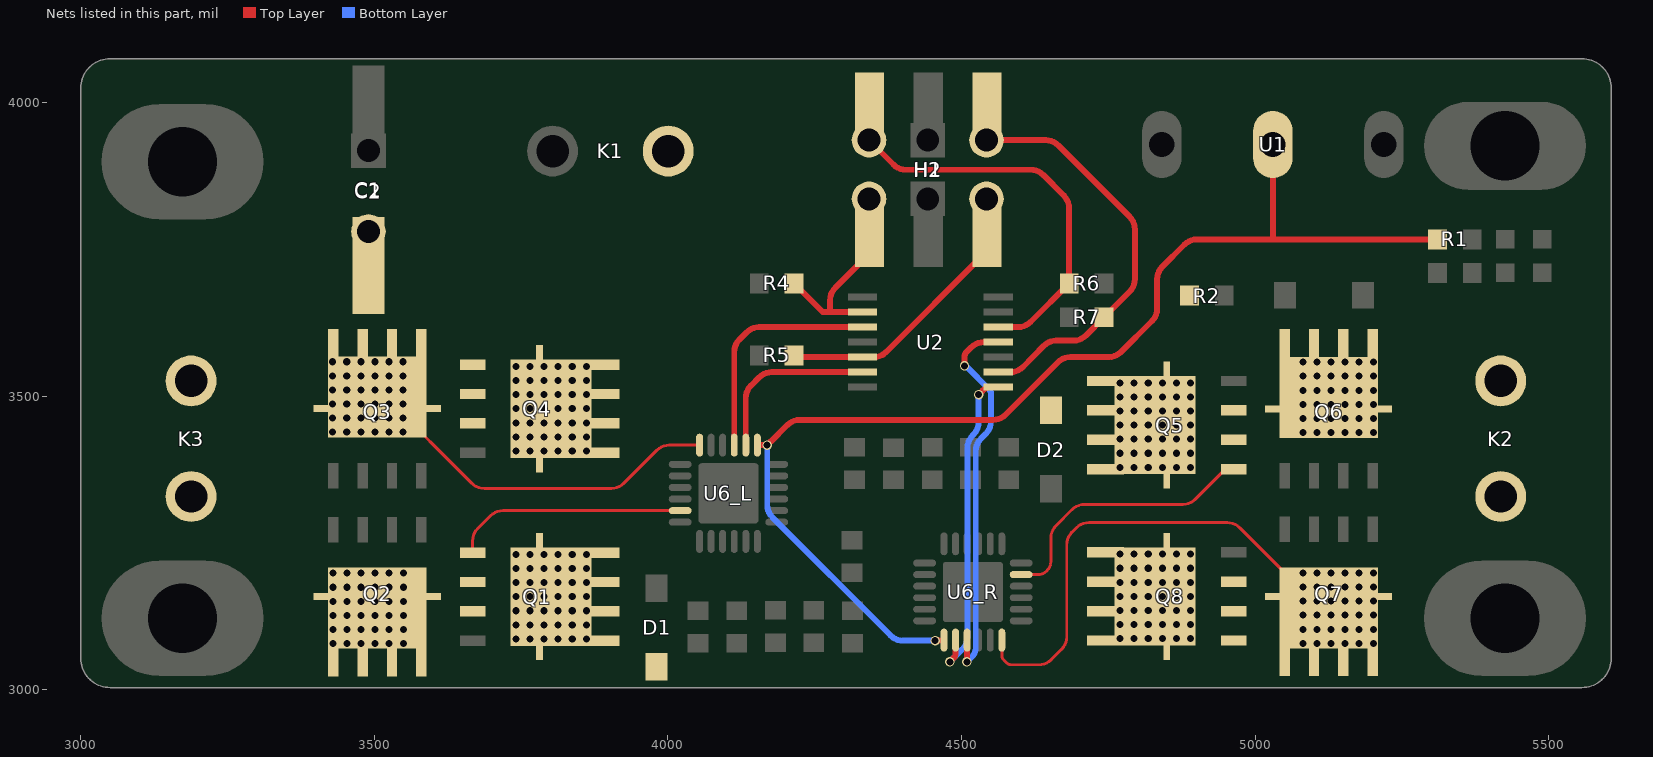
[diagram p0: the nets of this part, all layers, seen from the top]
# Altium PCB MISC62357.pcbdoc (part 2 of 2)
Units mil, origin at the board's own origin, x right, y up, seen from the top; angles counter-clockwise.
Board outline 2606.3 x 1070.87 mil, 2 copper layers (Top Layer, Bottom Layer), stack 62.206 mil thick; 46 components, 37 nets, 219 pads, 514 vias.

## Via types
v1: diameter 16, hole 12, Top Layer to Bottom Layer, 514 vias

## Nets (pads, with @x,y where several pads share a name; then routed paths per layer and width w, separated by ;. In a path a pad name is that pad's centre, name@x,y a point inside that pad or via, vN(x,y) a via of type N, cw(c..) or ccw(c..) an arc to the next point about the centre after c; other vN are vias at no path point) (continued)
L_A: K3.2 Q1.3 Q2.1 U6_L.23 | length 399.4
  Top Layer w5: Q1.3@3667.31,3233.6 3667.31,3253.49 cw(c3697.31,3253.49) 3676.1,3274.7 3697.69,3296.29 cw(c3718.9,3275.08) 3718.9,3305.08 U6_L.23@4020.8,3305.08
  other v1: 3429.35,3078.6 3453.35,3078.6 3477.35,3078.6 3501.35,3078.6 3525.35,3078.6 3549.35,3078.6 3429.35,3102.6 3453.35,3102.6 3477.35,3102.6 3501.35,3102.6 3525.35,3102.6 3549.35,3102.6 3429.35,3126.6 3453.35,3126.6 3477.35,3126.6 3501.35,3126.6 3525.35,3126.6 3549.35,3126.6 3429.35,3150.6 3453.35,3150.6 3477.35,3150.6 3501.35,3150.6 3525.35,3150.6 3549.35,3150.6 3429.35,3174.6 3453.35,3174.6 3477.35,3174.6 3501.35,3174.6 3525.35,3174.6 3549.35,3174.6 3429.35,3198.6 3453.35,3198.6 3477.35,3198.6 3501.35,3198.6 3525.35,3198.6 3549.35,3198.6
L_B: K3.1 Q3.1 Q4.3 U6_L.18 | length 639.5
  Top Layer w5: Q3.1@3505,3498.29 3515.17,3498.29 cw(c3515.17,3488.29) 3522.24,3495.36 3666.03,3351.57 ccw(c3687.24,3372.79) 3687.24,3342.79 3903.51,3342.79 ccw(c3903.51,3372.79) 3924.72,3351.57 3980.92,3407.77 cw(c4002.13,3386.56) 4002.13,3416.56 U6_L.18@4053.79,3416.56
  other v1: 3429,3438.6 3453,3438.6 3477,3438.6 3501,3438.6 3525,3438.6 3549,3438.6 3429,3462.6 3453,3462.6 3477,3462.6 3501,3462.6 3525,3462.6 3549,3462.6 3429,3486.6 3453,3486.6 3477,3486.6 3501,3486.6 3525,3486.6 3549,3486.6 3429,3510.6 3453,3510.6 3477,3510.6 3501,3510.6 3525,3510.6 3549,3510.6 3429,3534.6 3453,3534.6 3477,3534.6 3501,3534.6 3525,3534.6 3549,3534.6 3429,3558.6 3453,3558.6 3477,3558.6 3501,3558.6 3525,3558.6 3549,3558.6
L_DIR_IN: H1.1 H2.1 R4.1 U2.2 | length 294.4
  Top Layer w10: R4.1@4214.66,3692.07 4263.53,3643.21 4275.95,3643.21 ; U2.2@4331.32,3643.21 4275.95,3643.21 ; H1.1@4343.16,3775.44 4343.16,3755.18 cw(c4313.16,3755.18) 4334.37,3733.97 4284.74,3684.34 ccw(c4305.95,3663.13) 4275.95,3663.13 4275.95,3643.21
L_DIR_O: U2.3 U6_L.15 | length 399.3
  Top Layer w10: U6_L.15@4112.84,3416.56 4112.84,3575.01 cw(c4142.84,3575.01) 4121.63,3596.23 4134.23,3608.83 cw(c4155.44,3587.62) 4155.44,3617.62 U2.3@4331.32,3617.62
L_PWM_IN: H1.5 H2.5 R5.1 U2.5 | length 429.2
  Top Layer w10: R5.1@4214.73,3566.44 U2.5@4331.32,3566.44 4350.41,3566.44 ccw(c4350.41,3596.44) 4371.62,3575.22 4534.37,3737.97 ccw(c4513.16,3759.18) 4543.16,3759.18 H1.5@4543.16,3775.44
L_PWM_O: U2.6 U6_L.14 | length 301.9
  Top Layer w10: U6_L.14@4132.53,3416.56 4132.53,3496.7 cw(c4162.53,3496.7) 4141.32,3517.92 4155.46,3532.06 cw(c4176.67,3510.85) 4176.67,3540.85 U2.6@4331.32,3540.85
PWR_EN: R1.2 U1.2 U6_L.13 U6_R.13 | length 2002.7
  Top Layer w10: U6_L.13@4152.25,3416.6 4160.72,3416.6 ccw(c4160.72,3436.6) 4168.37,3418.12 ccw(c4160.72,3436.6) 4174.86,3422.46 4203.21,3450.81 cw(c4224.43,3429.6) 4224.43,3459.6 4553.57,3459.6 ccw(c4553.57,3489.6) 4574.79,3468.39 4664.21,3557.81 cw(c4685.43,3536.6) 4685.43,3566.6 4750.57,3566.6 ccw(c4750.57,3596.6) 4771.79,3575.39 4824.21,3627.81 ccw(c4803,3649.03) 4833,3649.03 4833,3699.17 cw(c4863,3699.17) 4841.79,3720.39 4879.5,3758.1 cw(c4900.72,3736.89) 4900.72,3766.89 5029.26,3766.89 ; v1(4455,3083.6) 4468.99,3083.6 U6_R.13@4470.03,3084.64 ; U1.2@5030.01,3928.47 5030.01,3767.63 5029.26,3766.89 ; R1.2@5310.34,3766.89 5029.26,3766.89
  Bottom Layer w10: v1(4169,3416.6) 4169,3315.03 ccw(c4199,3315.03) 4177.79,3293.81 4379.21,3092.39 ccw(c4400.43,3113.6) 4400.43,3083.6 v1(4455,3083.6)
R_A: K2.2 Q5.3 Q6.1 U6_R.23 | length 466.2
  Top Layer w5: U6_R.23@4601.44,3196.12 4630.24,3196.12 ccw(c4630.24,3216.12) 4644.38,3201.98 4646.13,3203.73 ccw(c4631.98,3217.87) 4651.98,3217.87 4651.98,3258.23 cw(c4681.98,3258.23) 4660.77,3279.44 4688.14,3306.81 cw(c4709.35,3285.6) 4709.35,3315.6 4876.57,3315.6 ccw(c4876.57,3345.6) 4897.79,3324.39 4946.23,3372.83 cw(c4953.3,3365.76) 4953.3,3375.76 Q5.3@4963.47,3375.76
  other v1: 5081,3437.97 5105,3437.97 5129,3437.97 5153,3437.97 5177,3437.97 5201,3437.97 5081,3461.97 5105,3461.97 5129,3461.97 5153,3461.97 5177,3461.97 5201,3461.97 5081,3485.97 5105,3485.97 5129,3485.97 5153,3485.97 5177,3485.97 5201,3485.97 5081,3509.97 5105,3509.97 5129,3509.97 5153,3509.97 5177,3509.97 5201,3509.97 5081,3533.97 5105,3533.97 5129,3533.97 5153,3533.97 5177,3533.97 5201,3533.97 5081,3557.97 5105,3557.97 5129,3557.97 5153,3557.97 5177,3557.97 5201,3557.97
R_B: K2.1 Q7.1 Q8.3 U6_R.18 | length 851.2
  Top Layer w5: U6_R.18@4568.45,3084.64 4568.45,3058.29 ccw(c4578.45,3058.29) 4571.38,3051.22 4577.06,3045.55 ccw(c4584.13,3052.62) 4584.13,3042.62 4631.59,3042.62 ccw(c4631.59,3072.62) 4652.8,3051.4 4670.24,3068.84 ccw(c4649.03,3090.06) 4679.03,3090.06 4679.03,3247.03 cw(c4709.03,3247.03) 4687.82,3268.24 4695.52,3275.94 cw(c4716.74,3254.73) 4716.74,3284.73 4952.44,3284.73 cw(c4952.44,3254.73) 4973.66,3275.94 4973.66,3275.75 5107.2,3142.21 5107.39,3142.21 ccw(c5114.47,3149.28) 5114.47,3139.28 Q7.1@5125,3139.28
  other v1: 5081,3078.96 5105,3078.96 5129,3078.96 5153,3078.96 5177,3078.96 5201,3078.96 5081,3102.96 5105,3102.96 5129,3102.96 5153,3102.96 5177,3102.96 5201,3102.96 5081,3126.96 5105,3126.96 5129,3126.96 5153,3126.96 5177,3126.96 5201,3126.96 5081,3150.96 5105,3150.96 5129,3150.96 5153,3150.96 5177,3150.96 5201,3150.96 5081,3174.96 5105,3174.96 5129,3174.96 5153,3174.96 5177,3174.96 5201,3174.96 5081,3198.96 5105,3198.96 5129,3198.96 5153,3198.96 5177,3198.96 5201,3198.96
R_DIR_IN: H1.2 H2.2 R6.2 U2.12 | length 671.2
  Top Layer w10: H2.2@4342.39,3935.88 4383.88,3894.39 ccw(c4405.1,3915.6) 4405.1,3885.6 4617.57,3885.6 cw(c4617.57,3855.6) 4638.79,3876.81 4674.21,3841.39 cw(c4653,3820.17) 4683,3820.17 4683,3692.2 R6.2@4683.13,3692.07 4617.47,3626.4 cw(c4596.26,3647.62) 4596.26,3617.62 U2.12@4561.64,3617.62
R_DIR_O: U2.11 U6_R.15 | length 657.9
  Top Layer w10: v1(4505,3551.6) 4505,3567.46 cw(c4515,3567.46) 4507.93,3574.53 4516.64,3583.24 cw(c4537.85,3562.03) 4537.85,3592.03 U2.11@4561.64,3592.03 ; v1(4509,3047.6) 4509,3084.24 U6_R.15@4509.4,3084.64
  Bottom Layer w10: v1(4505,3551.6) 4506.87,3551.6 4548,3510.47 4548,3508.6 4550,3506.6 4550,3457.03 cw(c4520,3457.03) 4541.21,3435.81 4532.79,3427.39 ccw(c4554,3406.17) 4524,3406.17 4524,3070.88 cw(c4504,3070.88) 4518.14,3056.74 v1(4509,3047.6)
R_PWM_IN: H1.6 H2.6 R7.2 U2.9 | length 709.1
  Top Layer w10: H2.6@4542.39,3935.88 4643.29,3935.88 cw(c4643.29,3905.88) 4664.51,3927.09 4786.21,3805.39 cw(c4765,3784.17) 4795,3784.17 4795,3699.34 cw(c4765,3699.34) 4786.21,3678.13 R7.2@4744.34,3636.26 ; U2.9@4561.64,3540.85 4583.15,3540.85 ccw(c4583.15,3570.85) 4604.51,3549.78 4639.9,3585.67 cw(c4661.26,3564.6) 4661.26,3594.6 4690.71,3594.6 ccw(c4690.71,3624.6) 4712.07,3603.53 R7.2@4742.45,3634.37 ; R7.2@4742.45,3634.37 R7.2@4744.34,3636.26 ; R7.2@4742.45,3634.37 R7.2@4744.34,3636.26
R_PWM_O: U2.8 U6_R.14 | length 549.1
  Top Layer w10: v1(4480,3047.6) 4486.78,3054.38 ccw(c4479.71,3061.45) 4489.71,3061.45 U6_R.14@4489.71,3084.64 ; v1(4529,3502.6) 4535.8,3509.4 cw(c4549.94,3495.26) 4549.94,3515.26 U2.8@4561.64,3515.26
  Bottom Layer w10: v1(4480,3047.6) 4501.2,3068.8 ccw(c4479.98,3090.01) 4509.98,3090.01 4509.98,3411.98 cw(c4539.98,3411.98) 4518.77,3433.19 4520.21,3434.63 ccw(c4499,3455.85) 4529,3455.85 v1(4529,3502.6)
VM: C1.1 C2.1 D1.2 D2.2 K1.1 Q1.1 Q4.1 Q5.1 Q8.1 R2.2
  other v1: 3741,3086.6 3765,3086.6 3789,3086.6 3813,3086.6 3837,3086.6 3861,3086.6 4769.79,3086.96 4793.79,3086.96 4817.79,3086.96 4841.79,3086.96 4865.79,3086.96 4889.79,3086.96 3741,3110.6 3765,3110.6 3789,3110.6 3813,3110.6 3837,3110.6 3861,3110.6 4769.79,3110.96 4793.79,3110.96 4817.79,3110.96 4841.79,3110.96 4865.79,3110.96 4889.79,3110.96 3741,3134.6 3765,3134.6 3789,3134.6 3813,3134.6 3837,3134.6 3861,3134.6 4769.79,3134.96 4793.79,3134.96 4817.79,3134.96 4841.79,3134.96 4865.79,3134.96 4889.79,3134.96 3741,3158.6 3765,3158.6 3789,3158.6 3813,3158.6 3837,3158.6 3861,3158.6 4769.79,3158.96 4793.79,3158.96 4817.79,3158.96 4841.79,3158.96 4865.79,3158.96 4889.79,3158.96 3741,3182.6 3765,3182.6 3789,3182.6 3813,3182.6 3837,3182.6 3861,3182.6 4769.79,3182.96 4793.79,3182.96 4817.79,3182.96 4841.79,3182.96 4865.79,3182.96 4889.79,3182.96 3741,3206.6 3765,3206.6 3789,3206.6 3813,3206.6 3837,3206.6 3861,3206.6 4769.79,3206.96 4793.79,3206.96 4817.79,3206.96 4841.79,3206.96 4865.79,3206.96 4889.79,3206.96 3741,3230.6 3765,3230.6 3789,3230.6 3813,3230.6 3837,3230.6 3861,3230.6 4769.79,3230.96 4793.79,3230.96 4817.79,3230.96 4841.79,3230.96 4865.79,3230.96 4889.79,3230.96 4769.79,3378.76 4793.79,3378.76 4817.79,3378.76 4841.79,3378.76 4865.79,3378.76 4889.79,3378.76 4769.79,3402.76 4793.79,3402.76 4817.79,3402.76 4841.79,3402.76 4865.79,3402.76 4889.79,3402.76 3741,3406.6 3765,3406.6 3789,3406.6 3813,3406.6 3837,3406.6 3861,3406.6 4769.79,3426.76 4793.79,3426.76 4817.79,3426.76 4841.79,3426.76 4865.79,3426.76 4889.79,3426.76 3741,3430.6 3765,3430.6 3789,3430.6 3813,3430.6 3837,3430.6 3861,3430.6 4769.79,3450.76 4793.79,3450.76 4817.79,3450.76 4841.79,3450.76 4865.79,3450.76 4889.79,3450.76 3741,3454.6 3765,3454.6 3789,3454.6 3813,3454.6 3837,3454.6 3861,3454.6 4769.79,3474.76 4793.79,3474.76 4817.79,3474.76 4841.79,3474.76 4865.79,3474.76 4889.79,3474.76 3741,3478.6 3765,3478.6 3789,3478.6 3813,3478.6 3837,3478.6 3861,3478.6 4769.79,3498.76 4793.79,3498.76 4817.79,3498.76 4841.79,3498.76 4865.79,3498.76 4889.79,3498.76 3741,3502.6 3765,3502.6 3789,3502.6 3813,3502.6 3837,3502.6 3861,3502.6 4769.79,3522.76 4793.79,3522.76 4817.79,3522.76 4841.79,3522.76 4865.79,3522.76 4889.79,3522.76 3741,3526.6 3765,3526.6 3789,3526.6 3813,3526.6 3837,3526.6 3861,3526.6 3741,3550.6 3765,3550.6 3789,3550.6 3813,3550.6 3837,3550.6 3861,3550.6
pads on no net: U6_L.9 U6_L.10 U6_L.11 U6_R.9 U6_R.10 U6_R.11

## Polygon pours and split planes (outlines as drawn)
VM on Top Layer (solid, remove dead copper, pour order 16): 3888.79,3989.85 3888.79,3714.75 4098.85,3714.75 4098.85,3989.85
VM on Bottom Layer (solid, remove dead copper, pour order 32): 3433,3830.6 3433,3739.6 3809,3739.6 3809,3830.6
VM on Bottom Layer (solid, remove dead copper, pour order 34): 3888.79,3989.85 3888.79,3730.75 4098.85,3730.75 4098.85,3989.85
VM on Top Layer (solid, remove dead copper, pour order 0): 3368.4,3830.59 3368.4,3644.33 3705.15,3644.33 3705.15,3393.67 3925.27,3393.67 3925.27,3830.59
L_A on Top Layer (solid, remove dead copper, pour order 2): 3074,3409.02 3351.58,3409.02 3406.57,3354.03 3406.57,3245.52 3416.5,3235.6 3593.14,3235.6 3643.14,3285.6 3699,3285.6 3699,3124.6 3683,3108.6 3642,3108.6 3629,3095.6 3629,3034.6 3616,3021.6 3422,3021.6 3396,3047.6 3338,3047.6 3312,3073.6 3312,3163.6 3253.77,3221.83 3074,3221.83
R_A on Top Layer (solid, remove dead copper, pour order 4): 5026,3620.6 5525.3,3620.6 5525.3,3432.07 5236.88,3432.07 5231.13,3427.56 5039.68,3427.56 5002,3389.87 5002,3363.6 4997,3358.6 4935,3358.6 4935,3491.6 4938,3494.6 4984,3494.6 4995,3505.6 4995,3589.6
R_B on Top Layer (solid, remove dead copper, pour order 6): 5525.68,3405.6 5525.68,3220.6 5345,3220.6 5287,3162.6 5287,3025.6 5284,3022.6 4967.51,3022.6 4929.57,3060.54 4929.57,3202.17 4932,3204.6 5015.23,3204.6 5033.57,3222.94 5197.46,3222.94 5231,3256.49 5231,3405.6
VM on Top Layer (solid, remove dead copper, pour order 8): 3748,3268.6 3912,3268.6 3933,3247.6 3933,3094.56 3949.86,3077.7 4014.27,3077.7 4014.27,3000 3955.6,3000 3936,3019.6 3936,3041.6 3929,3048.6 3738.55,3048.6 3726.98,3060.18 3726.98,3247.58
VM on Top Layer (solid, remove dead copper, pour order 10): 4849.3,3267.43 4726.83,3267.43 4706,3246.6 4706,3071.6 4727,3050.6 4894,3050.6 4907,3063.6 4907,3247.6 4887,3267.6 4849.47,3267.6
VM on Top Layer (solid, remove dead copper, pour order 12): 4854,3340.6 4716,3340.6 4700,3356.6 4700,3412.09 4685.35,3426.75 4628.42,3426.75 4618.42,3436.75 4618.42,3487.02 4667,3535.6 4816,3535.6 4864,3583.6 4864,3696.6 4863,3697.6 4900.87,3697.6 4907.53,3690.93 4907.53,3542.13 4899,3533.6 4899,3366.6 4880,3366.6
GND on Top Layer (solid, remove dead copper, pour order 18): 3050,4074.6 ccw(c3050,4024.6) 3000,4024.6 3000,3053.73 ccw(c3050,3053.73) 3050,3003.73 5556.3,3003.73 ccw(c5556.3,3053.73) 5606.3,3053.73 5606.3,4024.6 ccw(c5556.3,4024.6) 5556.3,4074.6
VM on Bottom Layer (solid, remove dead copper, pour order 20): 3726.98,3075.6 3928,3075.6 3928,3830.59 3706,3830.59 3706,3268.55 3726.98,3247.58
VM on Bottom Layer (solid, remove dead copper, pour order 22): 4909,3074.6 4712,3074.6 4712,3534.6 4713,3535.6 4646.81,3601.79 4038.17,3601.79 3928.98,3492.6 3899,3492.6 3899,3793.6 3896,3796.6 4815,3796.6 4909,3702.6
GND on Bottom Layer (solid, remove dead copper, pour order 36): 3050,4074.6 ccw(c3050,4024.6) 3000,4024.6 3000,3053.73 ccw(c3050,3053.73) 3050,3003.73 5556.3,3003.73 ccw(c5556.3,3053.73) 5606.3,3053.73 5606.3,4024.6 ccw(c5556.3,4024.6) 5556.3,4074.6
R_A on Bottom Layer (solid, remove dead copper, pour order 30): 5071.68,3616.6 5526.3,3616.6 5526.3,3432.07 5236.47,3432.07 5231.96,3427.56 5071.68,3427.56
R_B on Bottom Layer (solid, remove dead copper, pour order 28): 5526.68,3405.6 5526.68,3220.6 5345,3220.6 5287,3162.6 5287,3069.6 5071.57,3069.6 5071.57,3222.94 5197.46,3222.94 5231,3256.49 5231,3405.6
L_B on Bottom Layer (solid, remove dead copper, pour order 26): 3557.15,3626.6 3074,3626.6 3074,3430.75 3557.15,3430.75
L_A on Bottom Layer (solid, remove dead copper, pour order 24): 3074,3409.02 3351.58,3409.02 3406.57,3354.03 3406.57,3245.52 3416.5,3235.6 3558.14,3235.6 3558.14,3069.6 3316,3069.6 3312,3073.6 3312,3163.6 3253.77,3221.83 3074,3221.83
L_B on Top Layer (solid, remove dead copper, pour order 14): 3695,3626.6 3074,3626.6 3074,3430.75 3695,3430.75

## Keep-outs
Board Outline Layer:
  the board outline again, w10

## Other copper
Top Layer:
  region net AVDD_L: 4291.01,3149.46 4299.05,3155.56 4302.65,3153.29 4306.57,3151.62 4310.71,3150.6 4314.96,3150.26 4296.31,3133.55 4295.97,3137.8 4294.95,3141.93 4293.28,3145.86 4291.01,3149.46
  region net $1N3247: 4159.98,3146.55 4164.5,3156.17 4168.1,3153.9 4172.02,3152.23 4176.16,3151.21 4180.41,3150.87 4165.28,3130.64 4164.94,3134.89 4163.92,3139.02 4162.25,3142.95 4159.98,3146.55
  region net $1N3253: 4153.73,3095.13 4169.84,3107.3 4174.29,3103.88 4179.11,3101.01 4184.23,3098.73 4189.6,3097.08 4195.12,3096.08 4200.72,3095.75 4165.28,3064.25 4164.95,3069.85 4163.95,3075.37 4162.3,3080.73 4160.03,3085.86 4157.16,3090.68 4153.73,3095.13
  region net AVDD_R: 4340.9,3343.77 4333.55,3336.98 4329.94,3339.26 4326.02,3340.93 4321.88,3341.95 4317.64,3342.29 4335.6,3359.68 4335.94,3355.43 4336.96,3351.3 4338.63,3347.37 4340.9,3343.77
  region net $1N3253: 4048.79,3165.26 4058.79,3165.26 4059.11,3161.8 4060.06,3158.46 4061.62,3155.36 4063.72,3152.59 4066.29,3150.26 4041.29,3150.26 4043.86,3152.59 4045.96,3155.36 4047.51,3158.46 4048.47,3161.8 4048.79,3165.26
  region net $1N3253: 4099.04,3144.51 4099.04,3124.51 4091.37,3124.15 4083.77,3123.06 4076.3,3121.26 4069.04,3118.76 4069.04,3150.26 4076.3,3147.76 4083.77,3145.96 4091.37,3144.87 4099.04,3144.51
  region net $1N4036: 4573.45,3337.84 4563.45,3337.84 4563.25,3340.1 4562.65,3342.29 4581.45,3342.29 4579.09,3341.99 4576.87,3341.1 4574.95,3339.69 4573.45,3337.84
  region net $1N4036: 4628.08,3362.44 4628.08,3342.44 4613.08,3342.4 4598.08,3342.29 4598.08,3373.78 4602.38,3370.42 4607.06,3367.6 4612.04,3365.37 4617.26,3363.75 4622.63,3362.77 4628.08,3362.44
  region net $1N4036: 4532.65,3348.04 4532.65,3368.04 4540.32,3368.4 4547.92,3369.49 4555.39,3371.29 4562.65,3373.78 4562.65,3342.29 4555.39,3344.79 4547.92,3346.59 4540.32,3347.67 4532.65,3348.04
  region net $1N3022: 4225.1,3092.87 4231.06,3101.05 4234.67,3098.78 4238.59,3097.11 4242.73,3096.09 4246.97,3095.75 4230.4,3076.96 4230.06,3081.21 4229.04,3085.35 4227.38,3089.27 4225.1,3092.87
  region net $1N3253: 4152.09,3125.06 4140.7,3108.16 4135.98,3111.32 4130.94,3113.96 4125.65,3116.04 4120.17,3117.55 4114.56,3118.46 4108.88,3118.76 4134.86,3150.26 4138.27,3143.38 4142.3,3136.86 4146.92,3130.73 4152.09,3125.06
  region net $1N3253: 4069.43,3124.51 4069.43,3144.51 4077.1,3144.87 4084.7,3145.96 4092.17,3147.76 4099.43,3150.26 4099.43,3118.76 4092.17,3121.26 4084.7,3123.06 4077.1,3124.15 4069.43,3124.51
  region net $1N4031: 4395.61,3327.08 4383.29,3327.08 4379.89,3332.38 4375.91,3337.27 4371.4,3341.68 4396.4,3341.68 4394.59,3339.65 4393.38,3337.21 4392.87,3334.55 4393.09,3331.84 4394.03,3329.28 4395.61,3327.08
  region net $1N4029: 4406.81,3396.6 4397.77,3391.49 4394.16,3393.77 4390.24,3395.44 4386.11,3396.46 4381.86,3396.8 4401.5,3412.51 4401.85,3408.26 4402.87,3404.12 4404.53,3400.2 4406.81,3396.6
  region net $1N4036: 4480.97,3368.16 4493.03,3384.39 4497.75,3381.23 4502.79,3378.59 4508.08,3376.51 4513.56,3375 4519.17,3374.09 4524.85,3373.78 4497.53,3342.29 4495.14,3348 4492.27,3353.48 4488.93,3358.69 4485.16,3363.6 4480.97,3368.16
  region net $1N4036: 4562.96,3368.04 4562.96,3348.04 4555.29,3347.67 4547.69,3346.59 4540.22,3344.79 4532.96,3342.29 4532.96,3373.78 4540.22,3371.29 4547.69,3369.49 4555.29,3368.4 4562.96,3368.04
  region net $1N4034: 4473.14,3342.09 4464.1,3336.98 4460.5,3339.26 4456.58,3340.93 4452.44,3341.95 4448.19,3342.29 4467.84,3358 4468.18,3353.75 4469.2,3349.61 4470.87,3345.69 4473.14,3342.09
  region net $1N4036: 4479.39,3398.03 4463.28,3385.86 4458.84,3389.28 4454.02,3392.15 4448.89,3394.42 4443.53,3396.07 4438.01,3397.07 4432.41,3397.41 4467.84,3428.9 4468.17,3423.3 4469.17,3417.78 4470.82,3412.42 4473.1,3407.29 4475.97,3402.47 4479.39,3398.03
  region net $1N3253: 4010.11,3157.82 4000.89,3138.75 3996.17,3141.92 3991.13,3144.55 3985.84,3146.64 3980.36,3148.14 3974.75,3149.06 3969.07,3149.36 3999.51,3189.64 3999.81,3183.96 4000.72,3178.35 4002.23,3172.87 4004.31,3167.58 4006.95,3162.54 4010.11,3157.82
  region net $1N4036: 4603.18,3342.44 4603.18,3362.44 4613.25,3362.81 4623.27,3363.91 4633.18,3365.74 4633.18,3327.44 4629.95,3331.2 4626.24,3334.51 4622.14,3337.29 4617.7,3339.51 4613,3341.13 4608.14,3342.11 4603.18,3342.44
  region net $1N595: 5394.75,3704.97 5394.75,3714.97 5398.21,3715.29 5401.55,3716.25 5404.65,3717.8 5407.42,3719.9 5409.75,3722.47 5409.75,3697.47 5407.42,3700.05 5404.65,3702.15 5401.55,3703.7 5398.21,3704.65
  region net PWR_EN: 5279.46,3761.89 5279.46,3771.89 5282.92,3772.21 5286.26,3773.16 5289.37,3774.72 5292.13,3776.82 5294.46,3779.39 5294.46,3754.39 5292.13,3756.96 5289.37,3759.06 5286.26,3760.61 5282.92,3761.57 5279.46,3761.89
  region net $1N440: 5400.54,3771.89 5400.54,3761.89 5397.08,3761.57 5393.74,3760.61 5390.63,3759.06 5387.87,3756.96 5385.54,3754.39 5385.54,3779.39 5387.87,3776.82 5390.63,3774.72 5393.74,3773.16 5397.08,3772.21 5400.54,3771.89
  region net 3V6: 4978.18,3676.08 4978.18,3666.08 4974.73,3665.76 4971.39,3664.81 4968.28,3663.26 4965.51,3661.16 4963.18,3658.58 4963.18,3683.58 4965.51,3681.01 4968.28,3678.91 4971.39,3677.36 4974.73,3676.41 4978.18,3676.08
  region net 3V6: 5279.46,3704.87 5279.46,3714.87 5282.92,3715.19 5286.26,3716.15 5289.37,3717.7 5292.13,3719.8 5294.46,3722.37 5294.46,3697.37 5292.13,3699.95 5289.37,3702.05 5286.26,3703.6 5282.92,3704.55 5279.46,3704.87
  region net $1N595: 5400.54,3714.97 5400.54,3704.97 5397.08,3704.65 5393.74,3703.7 5390.63,3702.15 5387.87,3700.05 5385.54,3697.47 5385.54,3722.47 5387.87,3719.9 5390.63,3717.8 5393.74,3716.25 5397.08,3715.29 5400.54,3714.97
  region net L_DIR_IN: 4235.84,3677.96 4229.9,3669.76 4226.3,3672.03 4222.38,3673.7 4218.24,3674.72 4213.99,3675.06 4230.54,3693.87 4230.88,3689.62 4231.9,3685.48 4233.57,3681.56 4235.84,3677.96
  region net R_DIR_IN: 4667.89,3669.76 4661.96,3677.96 4664.23,3681.56 4665.9,3685.48 4666.92,3689.62 4667.26,3693.87 4683.8,3675.06 4679.56,3674.72 4675.42,3673.7 4671.5,3672.03 4667.89,3669.76
  region net R_DIR_IN: 4678,3724.08 4688,3724.08 4688.32,3720.62 4689.28,3717.28 4690.83,3714.17 4692.93,3711.41 4695.5,3709.08 4670.5,3709.08 4673.07,3711.41 4675.17,3714.17 4676.72,3717.28 4677.68,3720.62 4678,3724.08
  region net GND: 4726.94,3664.03 4713.93,3679.3 4717.57,3683.45 4720.66,3688.03 4723.14,3692.96 4724.97,3698.17 4726.13,3703.57 4726.58,3709.08 4758.33,3675.06 4752.69,3674.74 4747.12,3673.79 4741.69,3672.22 4736.48,3670.05 4731.54,3667.31 4726.94,3664.03
  region net R_PWM_IN: 4727.39,3611.95 4721.39,3620.1 4723.62,3623.73 4725.25,3627.66 4726.24,3631.8 4726.58,3636.05 4743.26,3617.36 4739.01,3617.01 4734.88,3615.97 4730.97,3614.27 4727.39,3611.95
  region net R_PWM_IN: 4757.69,3656.68 4763.63,3648.47 4761.36,3644.87 4759.69,3640.95 4758.67,3636.81 4758.33,3632.56 4741.78,3651.37 4746.03,3651.72 4750.17,3652.74 4754.09,3654.4 4757.69,3656.68
  region net GND: 4697.84,3663.22 4710.85,3647.94 4707.35,3643.59 4704.41,3638.84 4702.07,3633.76 4700.38,3628.43 4699.35,3622.94 4699.01,3617.36 4667.26,3651.37 4672.84,3651.72 4678.33,3652.75 4683.66,3654.44 4688.74,3656.77 4693.49,3659.71 4697.84,3663.22
  region net PWR_EN: 5035.01,3858.81 5025.01,3858.81 5024.91,3861.08 5024.61,3863.36 5024.1,3865.6 5023.34,3867.71 5022.32,3869.66 5021.02,3871.36 5019.42,3872.77 5017.51,3873.81 5042.51,3873.81 5040.59,3872.77 5038.99,3871.36 5037.69,3869.66 5036.67,3867.71 5035.91,3865.6 5035.4,3863.36 5035.1,3861.08
  region net 3V6: 5016.67,3666.08 5016.67,3676.08 5020.13,3676.41 5023.47,3677.36 5026.57,3678.91 5029.34,3681.01 5031.67,3683.58 5031.67,3658.58 5029.34,3661.16 5026.57,3663.26 5023.47,3664.81 5020.13,3665.76 5016.67,3666.08
  region net 3V6: 5071.24,3699.42 5074.37,3688.41 5072.1,3684.81 5070.43,3680.89 5069.41,3676.75 5069.07,3672.5 5055.33,3694.12 5059.58,3694.46 5063.72,3695.48 5067.64,3697.14 5071.24,3699.42
  region net $1N440: 5394.75,3761.89 5394.75,3771.89 5398.21,3772.21 5401.55,3773.16 5404.65,3774.72 5407.42,3776.82 5409.75,3779.39 5409.75,3754.39 5407.42,3756.96 5404.65,3759.06 5401.55,3760.61 5398.21,3761.57
  region net R_DIR_IN: 4374.43,3910.91 4367.36,3903.84 4365.72,3905.34 4364.15,3906.51 4362.65,3907.36 4361.19,3907.94 4359.76,3908.29 4358.34,3908.43 4355.45,3908.25 4349.01,3906.99 4345.18,3906.48 4343.04,3906.38 4340.75,3906.43 4371.84,3937.52 4371.89,3935.23 4371.79,3933.1 4371.28,3929.26 4370.03,3922.82 4369.84,3919.93 4369.98,3918.51 4370.33,3917.08 4370.91,3915.62 4371.76,3914.12 4372.93,3912.55
  region net R_PWM_IN: 4582.71,3940.88 4582.71,3930.88 4580.48,3930.78 4578.55,3930.5 4576.88,3930.04 4575.44,3929.42 4574.18,3928.65 4573.08,3927.75 4571.16,3925.57 4567.5,3920.13 4565.15,3917.06 4563.71,3915.48 4562.06,3913.89 4562.06,3957.87 4563.71,3956.28 4565.15,3954.7 4567.5,3951.63 4571.16,3946.19 4573.08,3944.02 4574.18,3943.11 4575.44,3942.34 4576.88,3941.72 4578.55,3941.26 4580.48,3940.98
  region net L_DIR_IN: 4322.49,3715.02 4312.85,3719.53 4315.13,3723.13 4316.8,3727.05 4317.82,3731.19 4318.16,3735.44 4338.4,3720.33 4334.16,3719.98 4330.02,3718.96 4326.1,3717.3 4322.49,3715.02
  region net L_PWM_IN: 4518.49,3715.02 4512.85,3723.53 4515.13,3727.13 4516.8,3731.05 4517.82,3735.19 4518.16,3739.44 4534.4,3720.33 4530.16,3719.98 4526.02,3718.96 4522.1,3717.3 4518.49,3715.02
  region net GL1_L: 3997.16,3381.31 3997.16,3386.31 4000.97,3387.56 4004.66,3389.13 4004.66,3378.48 4000.97,3380.05 3997.16,3381.31
  region net L_B: 4040.38,3414.06 4040.38,3419.06 4042.54,3419.31 4044.58,3420.05 4046.39,3421.23 4047.88,3422.81 4047.88,3410.31 4046.39,3411.88 4044.58,3413.07 4042.54,3413.81 4040.38,3414.06
  region net GH1_L: 4070.97,3436.99 4075.97,3436.99 4077.24,3434.75 4078.8,3432.7 4068.14,3432.7 4069.7,3434.75 4070.97,3436.99
  region net AVDD_L: 4208.51,3388.81 4208.51,3378.81 4203.63,3378.58 4198.79,3377.9 4198.79,3389.71 4203.63,3389.03 4208.51,3388.81
  region net GL2_R: 4625.08,3178.94 4625.08,3173.94 4621.27,3172.69 4617.58,3171.12 4617.58,3181.77 4621.27,3180.2 4625.08,3178.94
  region net GL1_R: 4624.87,3120.1 4625.28,3115.1 4621.45,3113.84 4617.78,3112.17 4617.37,3122.82 4621.08,3121.35 4624.87,3120.1
  region net PWR_EN: 4455,3078.6 4455,3088.6 4457.53,3088.95 4459.86,3089.97 4461.84,3091.59 4463.29,3093.69 4464.13,3096.1 4464.13,3071.1 4463.29,3073.51 4461.84,3075.61 4459.86,3077.23 4457.53,3078.25
  region net AVDD_R: 4408.45,3112.39 4408.45,3122.39 4415.96,3122.62 4423.45,3123.3 4423.45,3111.49 4415.96,3112.17 4408.45,3112.39
  region net L_DIR_IN: 4291.32,3638.21 4291.32,3648.21 4298.83,3648.46 4306.32,3649.21 4306.32,3637.21 4298.83,3637.96 4291.32,3638.21
  region net L_DIR_O: 4291.32,3612.62 4291.32,3622.62 4298.83,3622.87 4306.32,3623.62 4306.32,3611.62 4298.83,3612.37 4291.32,3612.62
  region net L_PWM_IN: 4291.32,3561.44 4291.32,3571.44 4298.83,3571.69 4306.32,3572.44 4306.32,3560.44 4298.83,3561.19 4291.32,3561.44
  region net L_PWM_IN: 4366.93,3577.67 4370.23,3567.59 4365.4,3565.6 4360.75,3563.21 4356.32,3560.44 4356.32,3572.44 4360.14,3573.55 4363.72,3575.31 4366.93,3577.67
  region net L_PWM_O: 4291.32,3535.85 4291.32,3545.85 4298.83,3546.1 4306.32,3546.85 4306.32,3534.85 4298.83,3535.6 4291.32,3535.85
  region net R_PWM_O: 4539.33,3505.86 4532.26,3512.93 4534.44,3515.44 4536.24,3518.24 4537.64,3521.26 4565.45,3509.26 4556.65,3508.88 4547.93,3507.74 4539.33,3505.86
  region net R_PWM_IN: 4598.75,3551.31 4601.87,3541.27 4596.93,3539.58 4592.17,3537.43 4587.64,3534.85 4587.64,3546.85 4591.61,3547.6 4595.36,3549.11 4598.75,3551.31
  region net R_DIR_O: 4522.67,3581.88 4522.67,3593.56 4527.8,3594.52 4532.81,3596.01 4537.64,3598.03 4537.64,3586.03 4533.66,3586.09 4529.75,3585.41 4526.04,3583.99 4522.67,3581.88
  region net R_DIR_IN: 4596.26,3622.62 4596.26,3612.62 4591.92,3612.36 4587.64,3611.62 4587.64,3623.62 4591.92,3622.87 4596.26,3622.62
  region net D3V3: 4537.62,3663.8 4537.62,3673.8 4537.63,3674.3 4537.64,3674.8 4537.64,3662.8 4537.63,3663.3 4537.62,3663.8
  region net L_A: 3664.81,3249.96 3669.81,3249.96 3670.06,3247.81 3670.8,3245.77 3671.99,3243.95 3673.56,3242.46 3661.06,3242.46 3662.64,3243.95 3663.82,3245.77 3664.56,3247.81 3664.81,3249.96
  region net GH2_L: 3687.97,3095.11 3691.62,3091.68 3690.17,3089.24 3689.27,3086.55 3688.97,3083.73 3680.02,3092.46 3682.84,3092.76 3685.53,3093.66 3687.97,3095.11
  region net GL2_L: 3436.94,3297.08 3441.51,3294.57 3440.06,3292.13 3439.16,3289.44 3438.86,3286.62 3428.99,3294.43 3431.81,3294.73 3434.5,3295.63 3436.94,3297.08
  region net L_B: 3591.31,3429.82 3587.33,3426.74 3584.89,3428.19 3582.2,3429.08 3579.37,3429.39 3588.66,3437.78 3588.97,3434.96 3589.86,3432.26 3591.31,3429.82
  region net L_B: 3522.9,3491.17 3532.68,3488.45 3534.67,3486.77 3536.91,3485.44 3539.34,3484.51 3526.84,3484.51 3525.91,3486.94 3524.58,3489.18 3522.9,3491.17
  region net L_B: 3555.1,3466.03 3545.32,3468.75 3543.33,3470.43 3541.09,3471.76 3538.66,3472.7 3551.16,3472.7 3552.09,3470.26 3553.42,3468.02 3555.1,3466.03
  region net GH1_L: 3691.62,3396.52 3688.97,3392.09 3686.53,3393.54 3683.84,3394.44 3681.02,3394.74 3688.97,3404.47 3689.27,3401.65 3690.17,3398.96 3691.62,3396.52
  region net R_A: 4941.18,3364.25 4939.17,3369.3 4940.62,3371.74 4941.52,3374.44 4941.82,3377.26 4949.14,3366.9 4946.32,3366.6 4943.62,3365.7 4941.18,3364.25
  region net GH2_R: 4943.19,3514.25 4939.17,3517.3 4940.62,3519.74 4941.52,3522.44 4941.82,3525.26 4951.14,3516.9 4948.32,3516.6 4945.62,3515.7 4943.19,3514.25
  region net GL2_R: 5192.78,3339.84 5188.49,3342.63 5189.94,3345.07 5190.84,3347.76 5191.14,3350.58 5200.73,3342.49 5197.91,3342.19 5195.22,3341.29 5192.78,3339.84
  region net GH1_R: 4939.17,3239.9 4940.66,3245.47 4943.1,3244.02 4945.8,3243.13 4948.62,3242.82 4941.82,3231.94 4941.52,3234.76 4940.62,3237.46 4939.17,3239.9
  region net R_DIR_O: 4500,3562.53 4510,3562.53 4509.92,3559.52 4510.18,3558.2 4510.96,3556.93 4499.04,3556.93 4499.82,3558.2 4500.08,3559.52
  region net PWR_EN: 4465.93,3088.6 4465.93,3078.6 4462.92,3078.68 4461.6,3078.42 4460.33,3077.64 4460.33,3089.56 4461.6,3088.78 4462.92,3088.52
  region net GND: 3580.93,3408.6 3580.93,3398.6 3577.92,3398.68 3576.6,3398.42 3575.33,3397.64 3575.33,3409.56 3576.6,3408.78 3577.92,3408.52
  region net L_B: 3520.48,3493.59 3524.85,3496.29 3525.9,3495.43 3527.16,3494.63 3529.61,3493.14 3517.99,3490.46 3518.69,3491.23 3519.69,3492.09 3520.47,3492.92 3520.6,3493.28
  region net L_B: 3534.69,3486.45 3535.63,3478.44 3534.96,3478.98 3534.18,3479.43 3532.38,3480.01 3530.52,3480.09 3529.64,3479.92 3528.86,3479.59 3531.54,3491.21 3533.03,3488.76 3533.83,3487.5
  region net L_B: 3540.84,3473.23 3548.85,3472.29 3549.9,3471.43 3551.16,3470.63 3553.61,3469.14 3541.99,3466.46 3542.32,3467.24 3542.49,3468.12 3542.41,3469.98 3541.83,3471.78 3541.38,3472.56
  region net L_B: 3558.69,3462.45 3559.63,3454.44 3558.96,3454.98 3558.18,3455.43 3556.38,3456.01 3554.52,3456.09 3553.64,3455.92 3552.86,3455.59 3555.54,3467.21 3557.03,3464.76 3557.83,3463.5
  region net GND: 4981.07,3728.6 4981.07,3738.6 4984.08,3738.52 4985.4,3738.78 4986.67,3739.56 4986.67,3727.64 4985.4,3728.42 4984.08,3728.68
  region net L_DIR_IN: 4270.95,3663.13 4270.63,3659.69 4269.69,3656.37 4268.15,3653.28 4266.07,3650.53 4263.53,3648.21 4275.95,3643.21 4290.95,3648.21 4288.15,3649.69 4285.7,3651.7 4283.68,3654.15 4282.19,3656.94 4281.26,3659.97 4280.95,3663.13 4270.95,3663.13
  region net PWR_EN: 5025.01,3801.89 5024.72,3796.54 5023.86,3791.25 5022.44,3786.08 5020.47,3781.09 5017.99,3776.34 5015.01,3771.89 5029.26,3766.89 5045.01,3771.89 5042.02,3776.34 5039.54,3781.09 5037.57,3786.08 5036.15,3791.25 5035.29,3796.54 5035.01,3801.89 5025.01,3801.89
  text "2026.4" at 5337.6,4008.66 h51.18
Bottom Layer:
  region net 3V6: 4846.02,3858.81 4836.02,3858.81 4835.93,3861.08 4835.63,3863.36 4835.12,3865.6 4834.36,3867.71 4833.34,3869.66 4832.04,3871.36 4830.44,3872.77 4828.52,3873.81 4853.52,3873.81 4851.61,3872.77 4850.01,3871.36 4848.71,3869.66 4847.69,3867.71 4846.93,3865.6 4846.42,3863.36 4846.12,3861.08
  region net D3V3: 4399.14,3191.6 4399.14,3201.6 4402.12,3201.53 4403.42,3201.79 4404.67,3202.56 4404.67,3190.64 4403.42,3191.41 4402.12,3191.68
  region net D3V3: 4338.27,3260.4 4331.2,3253.33 4329.12,3255.53 4328.01,3256.27 4326.55,3256.61 4334.99,3265.05 4335.33,3263.59 4336.07,3262.48
  region net D3V3: 4222.93,3310.08 4222.93,3300.08 4219.92,3300.16 4218.6,3299.9 4217.33,3299.11 4217.33,3311.04 4218.6,3310.25 4219.92,3309.99
  region net D3V3: 4285.73,3268.8 4292.8,3275.87 4294.88,3273.67 4295.99,3272.93 4297.45,3272.59 4289.01,3264.16 4288.67,3265.61 4287.93,3266.72
  region net D3V3: 4307.93,3269.6 4307.93,3259.6 4304.92,3259.68 4303.6,3259.42 4302.33,3258.64 4302.33,3270.56 4303.6,3269.78 4304.92,3269.52
  region net D3V3: 4386.8,3505.33 4379.73,3512.4 4381.93,3514.48 4382.67,3515.59 4383.01,3517.05 4391.45,3508.61 4389.99,3508.27 4388.88,3507.53
  region net R_DIR_O: 4516.45,3549.09 4510.78,3540.62 4509.65,3541.81 4508.57,3542.83 4507.37,3543.51 4506.67,3543.66 4505.88,3543.65 4512.8,3553.36 4513.36,3551.93 4514.18,3550.98 4515.23,3550.15
  region net R_PWM_O: 4484.2,3058.87 4491.27,3051.8 4489.07,3049.72 4488.33,3048.61 4487.99,3047.16 4479.55,3055.59 4481.01,3055.93 4482.12,3056.67
  region net PWR_EN: 4444.07,3078.6 4444.07,3088.6 4447.08,3088.52 4448.4,3088.78 4449.67,3089.56 4449.67,3077.64 4448.4,3078.42 4447.08,3078.68
  region net PWR_EN: 4174,3405.67 4164,3405.67 4164.08,3408.68 4163.82,3410 4163.04,3411.27 4174.96,3411.27 4174.18,3410 4173.92,3408.68
  region net 3V6: 4928,3695.53 4938,3695.53 4937.92,3692.52 4938.18,3691.2 4938.96,3689.93 4927.04,3689.93 4927.82,3691.2 4928.08,3692.52

## Silkscreen, mask and mechanical layers (free items; w line width, h text height)
Top Silkscreen Layer:
  text "R_DIR" at 4123,3909.6 h60
  text "R_PWM" at 4605.89,3909.6 h60
  text "L_DIR" at 4123,3781.6 h60
  text "L_PWM" at 4605.89,3781.6 h60
  text "GND" at 4415,3688.6 h40
  text "-" at 3754,3584.6 h200
  text "+" at 3953,3584.6 h200
Bottom Silkscreen Layer:
  text "GND" at 4252,3976.6 h60
  text "R_DIR" at 3883,3909.6 h60
  text "R_PWM" at 4365.89,3909.6 h60
  text "L_DIR" at 3883,3782.06 h60
  text "L_PWM" at 4365.89,3782.06 h60
  text "-" at 3854,3716.6 h200
  text "+" at 4048,3712.6 h200
Top Solder Mask Layer:
  text "COMPANY_A" at 3062.01,4010.62 h43.31
  text "2026.4" at 5336.61,4008.66 h51.18
  text "COMPANY_B" at 3034.45,3698.62 h35.43